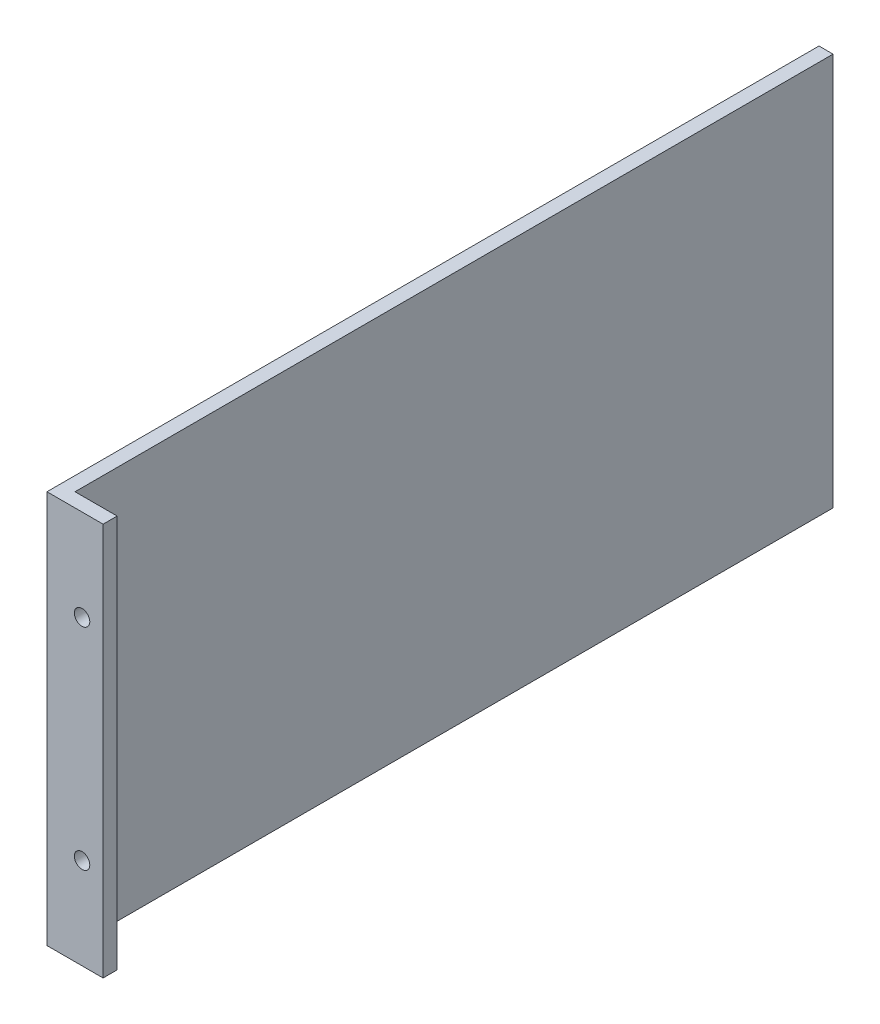
SolidWorks part; units mm, degrees
ref_plane "Front Plane" through (0, 0, 0) normal (0, 0, 1) x (1, 0, 0)
ref_plane "Top Plane" through (0, 0, 0) normal (0, 1, 0) x (1, 0, 0)
ref_plane "Right Plane" through (0, 0, 0) normal (1, 0, 0) x (0, 0, -1)
other "Configuration Table"
sketch "Sketch1" plane through (0, 0, 0) normal (0, 0, 1) x (1, 0, 0)
  line L0 (0, 0) -> (0, 470.1987) construction
  line L1 (360, 0) -> (-360, 0)
  line L2 (-360, 0) -> (-360, 20)
  line L3 (-360, 20) -> (-335, 20)
  line L4 (-335, 20) -> (-335, 580)
  line L5 (-335, 580) -> (-315, 580)
  line L6 (-315, 580) -> (-315, 20)
  line L7 (-315, 20) -> (315, 20)
  line L8 (315, 580) -> (315, 20)
  line L9 (335, 580) -> (315, 580)
  line L10 (335, 20) -> (335, 580)
  line L11 (360, 20) -> (335, 20)
  line L12 (360, 0) -> (360, 20)
  point P11 (0, 20)
  dimension "D1" = 720
  dimension "D2" = 560
  dimension "D3" = 20
  dimension "D4" = 20
  dimension "D5" = 315
extrude "Boss-Extrude1" add sketch "Sketch1" along normal blind 1100
sketch "Sketch2" plane through (0, 0, 0) normal (0, 0, -1) x (-1, 0, 0)
  line L0 (-360, 20) -> (-59.2408, 20)
  line L1 (-315, 20) -> (315, 20) construction
  line L2 (-59.2408, 20) -> (-59.2408, 755.063)
  line L3 (-59.2408, 755.063) -> (647.4274, 706.2518)
  line L4 (647.4274, 706.2518) -> (560.6518, -150.6574)
  line L5 (560.6518, -150.6574) -> (-360, -188.6217)
  line L6 (-360, -188.6217) -> (-684.0359, -70.6611)
  line L7 (-684.0359, -70.6611) -> (-360, 20)
extrude "Cut-Extrude1" cut sketch "Sketch2" against normal through all
sketch "Sketch3" plane through (335, 0, 0) normal (1, 0, 0) x (0, 0, -1)
  line L0 (-1100, 20) -> (0, 20) construction
  line L1 (-1100, 580) -> (-1080, 580)
  line L2 (-1100, 580) -> (-1100, 20)
  line L3 (-1100, 20) -> (-1080, 20)
  line L4 (-1080, 580) -> (-1080, 20)
  dimension "D1" = 20
extrude "Boss-Extrude2" add sketch "Sketch3" along normal blind 60
sketch "Sketch4" plane through (0, 0, 1080) normal (0, 0, -1) x (-1, 0, 0)
  line L0 (-395, 20) -> (-395, 580) construction
  line L1 (-395, 20) -> (-335, 20) construction
  circle A0 centre (-365, 450) radius 11
  circle A1 centre (-365, 150) radius 11
  dimension "D1" = 22
  dimension "D2" = 30
  dimension "D3" = 30
  dimension "D4" = 22
  dimension "D5" = 300
  dimension "D6" = 130
extrude "Cut-Extrude2" cut sketch "Sketch4" against normal through all
